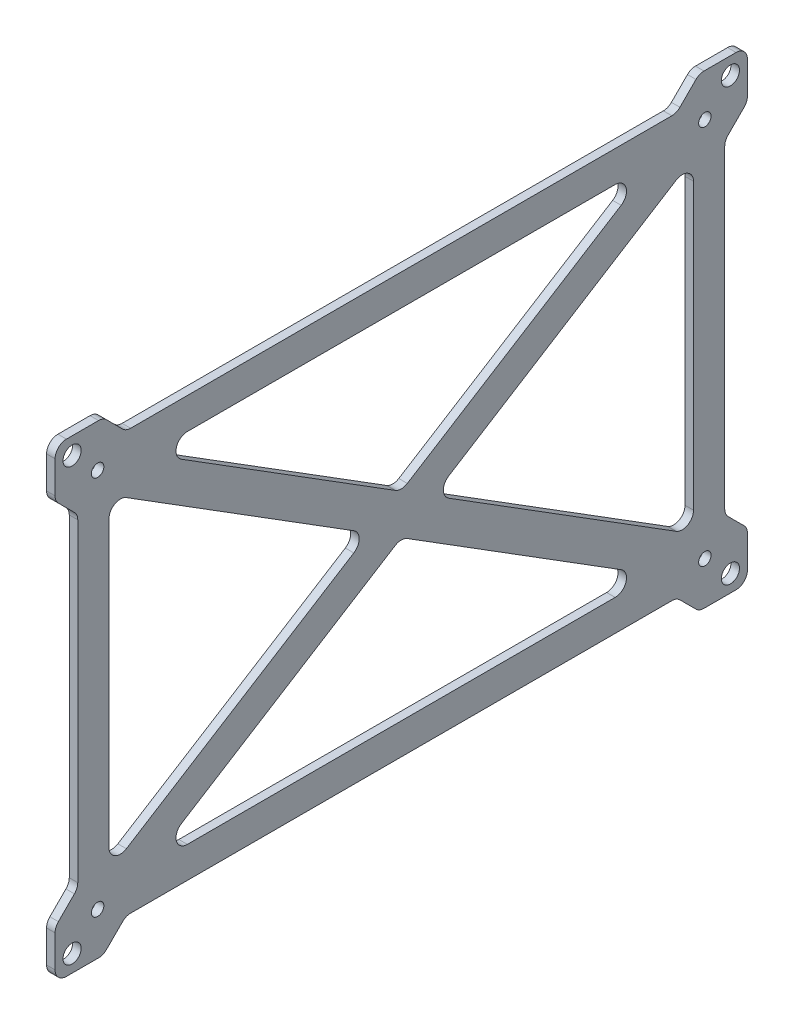
from build123d import *

# Parameters (mm, degrees)
SKETCH_1_W          = 122
SKETCH_1_H          = 82
SKETCH_1_R          = 1.6
SKETCH_1_R_2        = 1.1
EXTRUDE_1_DEPTH     = 1.5
CUT_EXTRUDE_1_DEPTH = 143.843445772
CUT_EXTRUDE_2_DEPTH = 143.843445772
FILLET_1_R          = 2


with BuildPart() as part:
    # 草图1 → 凸台-拉伸1 (new body)
    with BuildSketch(Plane(origin=(0, 0, 0), x_dir=(0, 0, -1), z_dir=(1, 0, 0))):
        with Locations((58, 38)):
            Rectangle(SKETCH_1_W, SKETCH_1_H)
        with Locations((0, 76)):
            Circle(SKETCH_1_R, mode=Mode.SUBTRACT)
        Circle(SKETCH_1_R, mode=Mode.SUBTRACT)
        with Locations((116, 76)):
            Circle(SKETCH_1_R, mode=Mode.SUBTRACT)
        with Locations((116, 0)):
            Circle(SKETCH_1_R, mode=Mode.SUBTRACT)
        with Locations((4.5, 71.5)):
            Circle(SKETCH_1_R_2, mode=Mode.SUBTRACT)
        with Locations((4.5, 4.5)):
            Circle(SKETCH_1_R_2, mode=Mode.SUBTRACT)
        with Locations((111.5, 71.5)):
            Circle(SKETCH_1_R_2, mode=Mode.SUBTRACT)
        with Locations((111.5, 4.5)):
            Circle(SKETCH_1_R_2, mode=Mode.SUBTRACT)
    extrude(amount=EXTRUDE_1_DEPTH)

    # 草图2 → 切除-拉伸1 (cut, through all)
    with BuildSketch(Plane(origin=(1.5, 0, 0), x_dir=(0, 0, -1), z_dir=(1, 0, 0))):
        Polygon((102.653173492, 69.5), (13.346826508, 69.5), (58, 41.539601645), align=None)
        Polygon((52.347203343, 38), (6.5, 66.708061906), (6.5, 9.291938094), align=None)
        Polygon((102.653173492, 6.5), (58, 34.460398355), (13.346826508, 6.5), align=None)
        Polygon((109.5, 66.708061906), (63.652796657, 38), (109.5, 9.291938094), align=None)
    extrude(amount=-CUT_EXTRUDE_1_DEPTH, mode=Mode.SUBTRACT)

    # 草图3 → 切除-拉伸2 (cut, through all)
    with BuildSketch(Plane(origin=(1.5, 0, 0), x_dir=(0, 0, -1), z_dir=(1, 0, 0))):
        Polygon((5.485281374, 79), (9.485281374, 75), (106.514718626, 75), (110.514718626, 79), align=None)
        Polygon((106.514718626, 1), (110.514718626, -3), (5.485281374, -3), (9.485281374, 1), align=None)
        Polygon((-3, 70.514718626), (1, 66.514718626), (1, 9.485281374), (-3, 5.485281374), align=None)
        Polygon((115, 9.485281374), (119, 5.485281374), (119, 70.514718626), (115, 66.514718626), align=None)
    extrude(amount=-CUT_EXTRUDE_2_DEPTH, mode=Mode.SUBTRACT)

    # 圆角1
    fillet_1_edges = [part.edges().sort_by_distance(p)[0] for p in [
        (0.75, 79, -5.485281374),
        (0.75, 79, -110.514718626),
        (0.75, 75, -106.514718626),
        (0.75, 75, -9.485281374),
        (0.75, 1, -9.485281374),
        (0.75, 1, -106.514718626),
        (0.75, -3, -110.514718626),
        (0.75, -3, -5.485281374),
        (0.75, 5.485281374, 3),
        (0.75, 70.514718626, 3),
        (0.75, 66.514718626, -1),
        (0.75, 9.485281374, -1),
        (0.75, 9.485281374, -115),
        (0.75, 66.514718626, -115),
        (0.75, 70.514718626, -119),
        (0.75, 5.485281374, -119),
        (0.75, 6.5, -102.653173492),
        (0.75, 6.5, -13.346826508),
        (0.75, 34.460398355, -58),
        (0.75, 9.291938094, -6.5),
        (0.75, 66.708061906, -6.5),
        (0.75, 38, -52.347203343),
        (0.75, 66.708061906, -109.5),
        (0.75, 9.291938094, -109.5),
        (0.75, 38, -63.652796657),
        (0.75, 69.5, -102.653173492),
        (0.75, 41.539601645, -58),
        (0.75, 69.5, -13.346826508),
        (0.75, 79, 3),
        (0.75, 79, -119),
        (0.75, -3, -119),
        (0.75, -3, 3),
    ]]
    fillet(fillet_1_edges, radius=FILLET_1_R)


solid = part.part
